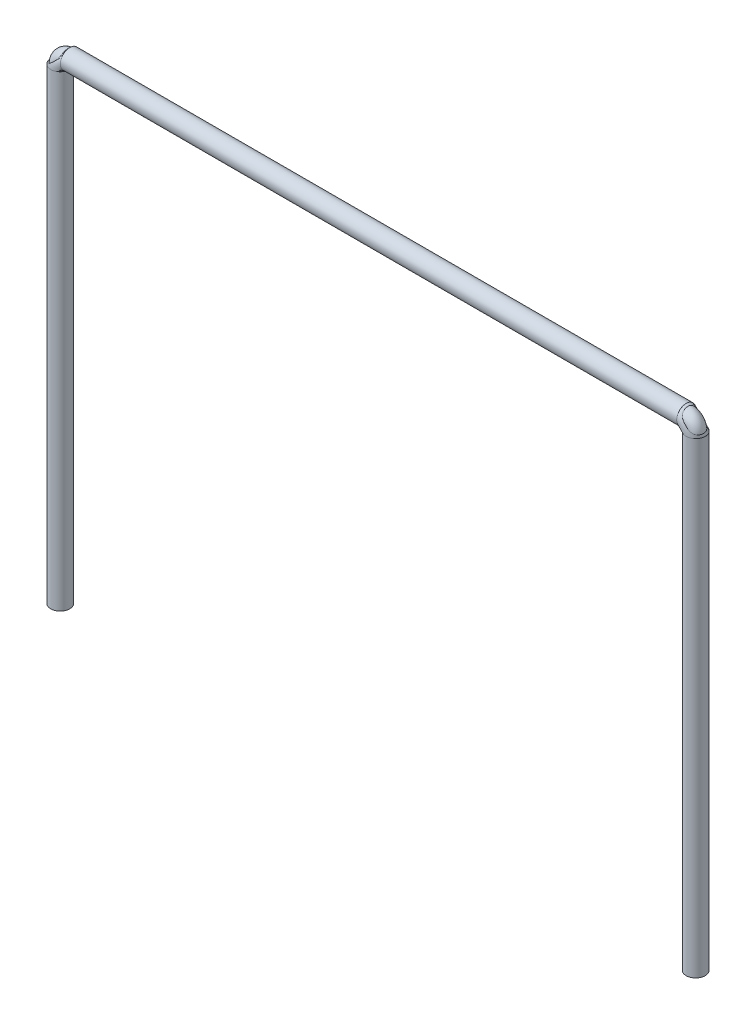
SolidWorks part; units mm, degrees
ref_plane "Front Plane" through (0, 0, 0) normal (0, 0, 1) x (1, 0, 0)
ref_plane "Top Plane" through (0, 0, 0) normal (0, 1, 0) x (1, 0, 0)
ref_plane "Right Plane" through (0, 0, 0) normal (1, 0, 0) x (0, 0, -1)
other "Configuration Table"
sketch3d "3DSketch1"
  line L0 (0, 0, 0) -> (0, 836.0539, 0) construction
  line L1 (0, 0, 0) -> (0, 1470, 0)
  line L2 (30, 1500, 0) -> (1970, 1500, 0)
  line L3 (2000, 1470, 0) -> (2000, 0, 0)
  arc A0 (2000, 1470, 0) -> (1970, 1500, 0) centre (1970, 1470, 0) ccw
  arc A1 (0, 1470, 0) -> (30, 1500, 0) centre (30, 1470, 0) ccw
  point P8 (2000, 1500, 0)
  point P9 (1970, 1470, 30)
  point P12 (0, 1500, 0)
  point P13 (30, 1470, -30)
  dimension "D4" = 30
  dimension "D1" = 1500
  dimension "D2" = 2000
  dimension "D3" = 1500
other "Gb／t6728-2002 round tube 060 X 5 (1)"
ref_plane "Plane1" through (0, 0, 0) normal (0, 1, 0) x (1, 0, 0)
sketch "Sketch1" plane through (0, 0, 0) normal (0, 1, 0) x (1, 0, 0)
  circle A0 centre (0, 0) radius 25
  circle A1 centre (0, 0) radius 30
  point P3 (0, 0)
  dimension "Out_dia" = 60
  dimension "D1" = 5
